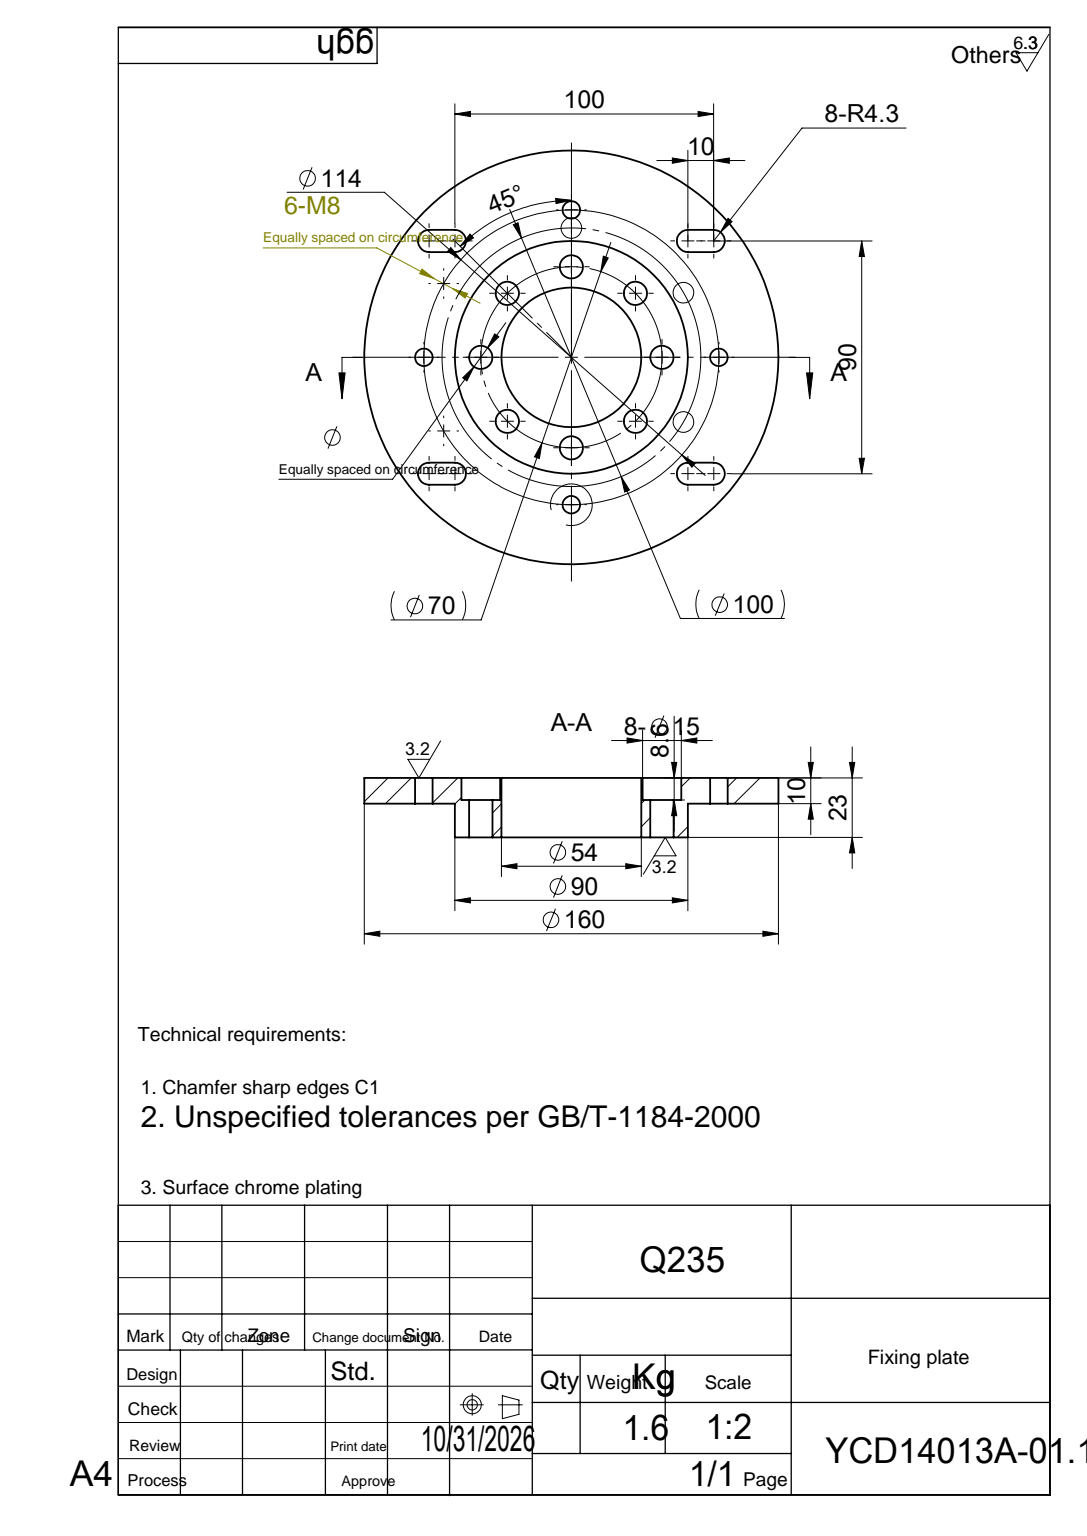
from build123d import *

# Parameters (mm, degrees)
SKETCH1_R                                           = 45
SKETCH1_R_2                                         = 27
BOSS_EXTRUDE1_DEPTH                                 = 13
SKETCH2_R                                           = 80
BOSS_EXTRUDE2_DEPTH                                 = 10
CUT_EXTRUDE1_DEPTH                                  = 114.881517377
CIRPATTERN1_COUNT                                   = 4
SKETCH6_R                                           = 27
CUT_EXTRUDE2_DEPTH                                  = 114.881517377
CBORE_FOR_M8_HEX_SOCKET_HEAD_CAP_SCREW1_D           = 9
CBORE_FOR_M8_HEX_SOCKET_HEAD_CAP_SCREW1_CBORE_D     = 15
CBORE_FOR_M8_HEX_SOCKET_HEAD_CAP_SCREW1_CBORE_DEPTH = 8.6
CIRPATTERN2_COUNT                                   = 8


with BuildPart() as part:
    # Sketch1 → Boss-Extrude1 (new body)
    with BuildSketch(Plane.XY):
        with Locations(Location((0, 0, 0), (0, 0, 180))):
            Circle(SKETCH1_R)
        with Locations(Location((0, 0, 0), (0, 0, 180))):
            Circle(SKETCH1_R_2, mode=Mode.SUBTRACT)
    extrude(amount=BOSS_EXTRUDE1_DEPTH)

    # Sketch2 → Boss-Extrude2 (add)
    with BuildSketch(Plane.XY):
        Circle(SKETCH2_R)
    extrude(amount=-BOSS_EXTRUDE2_DEPTH)

    # Sketch3 → M8 Tapped Hole1 (revolve, cut)
    with BuildSketch(Plane(origin=(0, -57, 0), x_dir=(0, -1, 0), z_dir=(1, 0, 0))):
        Polygon((0, 0), (0, 24.342926105), (3.4, 22.3), (3.4, 0), align=None)
    m8_tapped_hole1 = revolve(axis=Axis((0, -57, 6.35), (0, 0, -1)), mode=Mode.SUBTRACT)

    # Sketch5 → Cut-Extrude1 (cut, through all)
    with BuildSketch(Plane.XY):
        with BuildLine():
            Line((45, 49.271909465), (55, 49.271909465))
            ThreePointArc((55, 49.271909465), (59.271909465, 45), (55, 40.728090535))
            Line((55, 40.728090535), (45, 40.728090535))
            ThreePointArc((45, 40.728090535), (40.728090535, 45), (45, 49.271909465))
        make_face()
        with BuildLine():
            Line((45, -40.728090535), (55, -40.728090535))
            ThreePointArc((55, -40.728090535), (59.271909465, -45), (55, -49.271909465))
            Line((55, -49.271909465), (45, -49.271909465))
            ThreePointArc((45, -49.271909465), (40.728090535, -45), (45, -40.728090535))
        make_face()
        with BuildLine():
            Line((-45, -40.728090535), (-55, -40.728090535))
            ThreePointArc((-55, -40.728090535), (-59.271909465, -45), (-55, -49.271909465))
            Line((-55, -49.271909465), (-45, -49.271909465))
            ThreePointArc((-45, -49.271909465), (-40.728090535, -45), (-45, -40.728090535))
        make_face()
        with BuildLine():
            Line((-45, 49.271909465), (-55, 49.271909465))
            ThreePointArc((-55, 49.271909465), (-59.271909465, 45), (-55, 40.728090535))
            Line((-55, 40.728090535), (-45, 40.728090535))
            ThreePointArc((-45, 40.728090535), (-40.728090535, 45), (-45, 49.271909465))
        make_face()
    extrude(amount=-CUT_EXTRUDE1_DEPTH, mode=Mode.SUBTRACT)

    # CirPattern1: M8 Tapped Hole1 ×4 about axis
    cirpattern1_axis = Axis((0, 0, 0), (0, 0, 1))
    for i in range(1, CIRPATTERN1_COUNT):
        add(m8_tapped_hole1.rotate(cirpattern1_axis, i * 360 / CIRPATTERN1_COUNT), mode=Mode.SUBTRACT)

    # Sketch6 → Cut-Extrude2 (cut, through all)
    with BuildSketch(Plane.XY):
        with Locations(Location((0, 0, 0), (0, 0, 180))):
            Circle(SKETCH6_R)
    extrude(amount=-CUT_EXTRUDE2_DEPTH, mode=Mode.SUBTRACT)

    # CBORE for M8 Hex Socket Head Cap Screw1 (through all)
    with Locations(Plane(origin=(0, 0, -10), x_dir=(-1, 0, 0), z_dir=(0, 0, -1))):
        with Locations((35, 0)):
            cbore_for_m8_hex_socket_head_cap_screw1 = CounterBoreHole(CBORE_FOR_M8_HEX_SOCKET_HEAD_CAP_SCREW1_D / 2, CBORE_FOR_M8_HEX_SOCKET_HEAD_CAP_SCREW1_CBORE_D / 2, CBORE_FOR_M8_HEX_SOCKET_HEAD_CAP_SCREW1_CBORE_DEPTH)

    # CirPattern2: CBORE for M8 Hex Socket Head Cap Screw1 ×8 about axis
    cirpattern2_axis = Axis((0, 0, 0), (0, 0, 1))
    for i in range(1, CIRPATTERN2_COUNT):
        add(cbore_for_m8_hex_socket_head_cap_screw1.rotate(cirpattern2_axis, i * 360 / CIRPATTERN2_COUNT), mode=Mode.SUBTRACT)


solid = part.part
